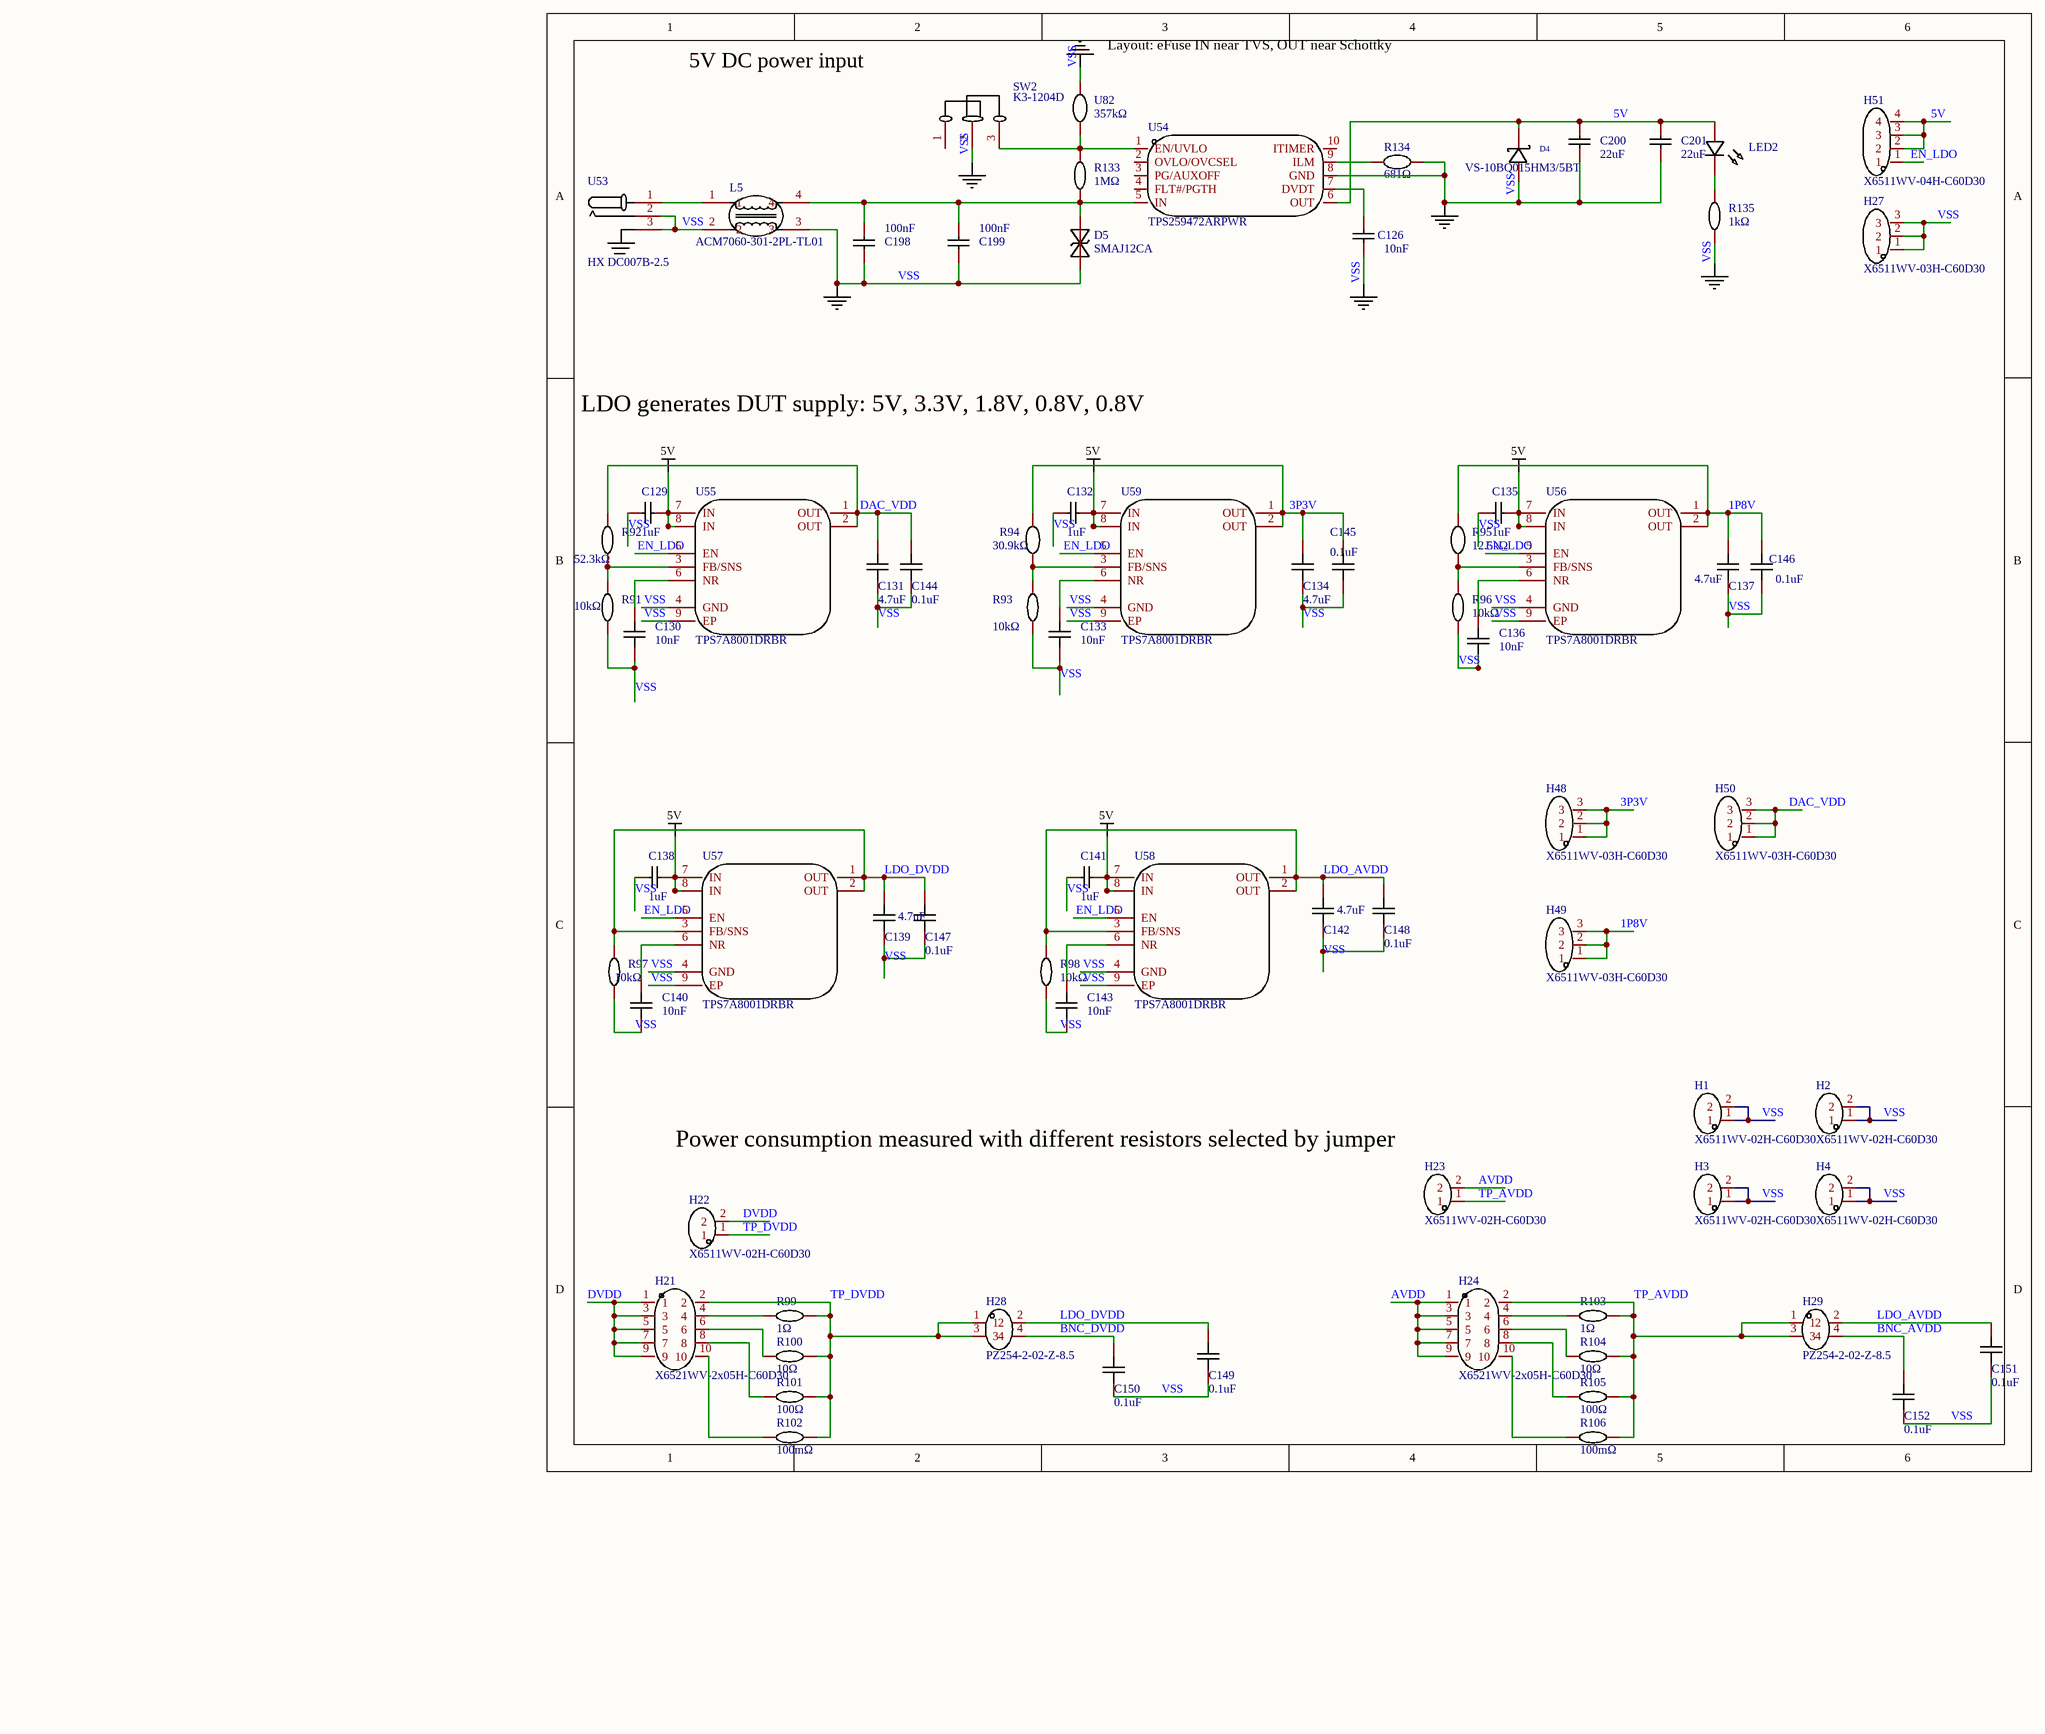
[diagram p0: MISC62793-2.schdoc]
# Altium project MISC62793-14.PrjPcb (part 1 of 4)
4 sheets, 201 parts. Net scope: global (net labels, ports and power ports of the same name join across sheets).
Board file: MISC62793.pcbdoc
Sheets:
  MISC62793-2.schdoc
  MISC62793-4.schdoc
  MISC62793-6.schdoc
  MISC62793-8.schdoc

## Sheet MISC62793-2.schdoc
size 279 x 274 mm; SheetNumber: 1; SheetTotal: 4

### Parts
C126  10nF  [C0603]
C129  1uF  [C0603]
C130  10nF  [C0603]
C131  4.7uF  [C0805]
C132  1uF  [C0603]
C133  10nF  [C0603]
C134  4.7uF  [C0805]
C135  1uF  [C0603]
C136  10nF  [C0603]
C137  4.7uF  [C0805]
C138  1uF  [C0603]
C139  4.7uF  [C0805]
C140  10nF  [C0603]
C141  1uF  [C0603]
C142  4.7uF  [C0805]
C143  10nF  [C0603]
C144  0.1uF  [C0402]
C145  0.1uF  [C0402]
C146  0.1uF  [C0402]
C147  0.1uF  [C0402]
C148  0.1uF  [C0402]
C149  0.1uF  [C0402]
C150  0.1uF  [C0402]
C151  0.1uF  [C0402]
C152  0.1uF  [C0402]
C198  100nF  [C0402]
C199  100nF  [C0402]
C200  22uF  [C1206]
C201  22uF  [C1206]
D4  VS-10BQ015HM3/5BT  [SMB_L4.6-W3.6-LS5.3-RD]
D5  SMAJ12CA  [SMA_L4.2-W2.7-LS5.0-BI]
H1  X6511WV-02H-C60D30  [HDR-TH_2P-P2.54-V-M]
H2  X6511WV-02H-C60D30  [HDR-TH_2P-P2.54-V-M]
H3  X6511WV-02H-C60D30  [HDR-TH_2P-P2.54-V-M]
H4  X6511WV-02H-C60D30  [HDR-TH_2P-P2.54-V-M]
H21  X6521WV-2x05H-C60D30  [HDR-TH_10P-P2.54-V-M-R2-C5-S2.54]
H22  X6511WV-02H-C60D30  [HDR-TH_2P-P2.54-V-M]
H23  X6511WV-02H-C60D30  [HDR-TH_2P-P2.54-V-M]
H24  X6521WV-2x05H-C60D30  [HDR-TH_10P-P2.54-V-M-R2-C5-S2.54]
H27  X6511WV-03H-C60D30  [HDR-TH_3P-P2.54-V-M]
H28  PZ254-2-02-Z-8.5  [HDR-TH_4P-P2.54-V-M-R2-C2-S2.54]
H29  PZ254-2-02-Z-8.5  [HDR-TH_4P-P2.54-V-M-R2-C2-S2.54]
H48  X6511WV-03H-C60D30  [HDR-TH_3P-P2.54-V-M]
H49  X6511WV-03H-C60D30  [HDR-TH_3P-P2.54-V-M]
H50  X6511WV-03H-C60D30  [HDR-TH_3P-P2.54-V-M]
H51  X6511WV-04H-C60D30  [HDR-TH_4P-P2.54-V-M]
L5  ACM7060-301-2PL-TL01  [FILTER-SMD_4P-L7.0-W6.0-TL_SMCM7060]
LED2  LED_0805-R  [LED_0805]  (value not drawn)
R91  10kΩ  [R0603]
R92  52.3kΩ  [R0603]
R93  10kΩ  [R0603]
R94  30.9kΩ  [R0603]
R95  12.5kΩ  [R0603]
R96  10kΩ  [R0603]
R97  10kΩ  [R0603]
R98  10kΩ  [R0603]
R99  1Ω  [R1206]
R100  10Ω  [R1206]
R101  100Ω  [R1206]
R102  100mΩ  [R1206]
R103  1Ω  [R1206]
R104  10Ω  [R1206]
R105  100Ω  [R1206]
R106  100mΩ  [R1206]
R133  1MΩ  [R1206]
R134  681Ω  [R0603]
R135  1kΩ  [R0805]
SW2  K3-1204D  [SW-TH_K3-1204D]
U53  HX DC007B-2.5  [DC-IN-TH_HX-DC007B-2.5]
U54  TPS259472ARPWR  [VQFN-10_L2.0-W2.0-P0.45-TL]
U55  TPS7A8001DRBR  [VSON-8_L3.0-W3.0-P0.65-TL-EP]
U56  TPS7A8001DRBR  [VSON-8_L3.0-W3.0-P0.65-TL-EP]
U57  TPS7A8001DRBR  [VSON-8_L3.0-W3.0-P0.65-TL-EP]
U58  TPS7A8001DRBR  [VSON-8_L3.0-W3.0-P0.65-TL-EP]
U59  TPS7A8001DRBR  [VSON-8_L3.0-W3.0-P0.65-TL-EP]
U82  357kΩ  [R1206]

### Nets
5V: C129.2 C132.2 C135.2 C138.2 C141.2 C200.2 C201.2 D4.1(C) H51.2 H51.3 H51.4 LED2.2(A) U54.6(OUT) U55.7(IN) U55.8(IN) U56.7(IN) U56.8(IN) U57.7(IN) U57.8(IN) U58.7(IN) U58.8(IN) U59.7(IN) U59.8(IN)
VSS: C126.1 C129.1 C130.1 C131.1 C132.1 C133.1 C134.1 C135.1 C136.1 C137.1 C138.1 C139.1 C140.1 C141.1 C142.1 C143.1 C144.1 C145.1 C146.1 C147.1 C148.1 C149.1 C150.1 C151.1 C152.1 C198.1 C199.1 C200.1 C201.1 D4.2(A) D5.1 H1.1 H1.2 H2.1 H2.2 H3.1 H3.2 H4.1 H4.2 H27.1 H27.2 H27.3 L5.2 L5.3 R91.1 R93.1 R96.1 R97.1 R98.1 R134.2 R135.1 SW2.2 U53.2 U53.3 U54.8(GND) U55.4(GND) U55.9(EP) U56.4(GND) U56.9(EP) U57.4(GND) U57.9(EP) U58.4(GND) U58.9(EP) U59.4(GND) U59.9(EP) U82.2
1P8V: C137.2 C146.2 H49.1 H49.2 H49.3 R95.2 U56.1(OUT) U56.2(OUT)
3P3V: C134.2 C145.2 H48.1 H48.2 H48.3 R94.1 U59.1(OUT) U59.2(OUT)
AVDD: H23.2 H24.1 H24.3 H24.5 H24.7 H24.9
BNC_AVDD: C152.2 H29.4
BNC_DVDD: C150.2 H28.4
DAC_VDD: C131.2 C144.2 H50.1 H50.2 H50.3 R92.2 U55.1(OUT) U55.2(OUT)
DVDD: H21.1 H21.3 H21.5 H21.7 H21.9 H22.2
EN_LDO: H51.1 U55.5(EN) U56.5(EN) U57.5(EN) U58.5(EN) U59.5(EN)
LDO_AVDD: C142.2 C148.2 C151.2 H29.2 R98.2 U58.1(OUT) U58.2(OUT) U58.3(FB/SNS)
LDO_DVDD: C139.2 C147.2 C149.2 H28.2 R97.2 U57.1(OUT) U57.2(OUT) U57.3(FB/SNS)
TP_AVDD: H23.1 H24.2 H29.1 H29.3 R103.2 R104.2 R105.2 R106.2
TP_DVDD: H21.2 H22.1 H28.1 H28.3 R99.2 R100.2 R101.2 R102.2
NetC126_2: C126.2 U54.7(DVDT)
NetC130_2: C130.2 U55.6(NR)
NetC133_2: C133.2 U59.6(NR)
NetC136_2: C136.2 U56.6(NR)
NetC140_2: C140.2 U57.6(NR)
NetC143_2: C143.2 U58.6(NR)
NetC198_2: C198.2 C199.2 D5.2 L5.4 R133.1 U54.5(IN)
NetH21_4: H21.4 R99.1
NetH21_6: H21.6 R100.1
NetH21_8: H21.8 R101.1
NetH21_10: H21.10 R102.1
NetH24_4: H24.4 R103.1
NetH24_6: H24.6 R104.1
NetH24_8: H24.8 R105.1
NetH24_10: H24.10 R106.1
NetL5_1: L5.1 U53.1
NetLED2_1: LED2.1(C) R135.2
NetR91_2: R91.2 R92.1 U55.3(FB/SNS)
NetR93_2: R93.2 R94.2 U59.3(FB/SNS)
NetR95_1: R95.1 R96.2 U56.3(FB/SNS)
NetR133_2: R133.2 SW2.3 U54.1(EN/UVLO) U82.1
NetR134_1: R134.1 U54.9(ILM)

Not connected (* = marked no-connect by the designer): SW2 1; U54 2(OVLO/OVCSEL) 3(PG/AUXOFF) 4(FLT#/PGTH) 10(ITIMER)

### Notes on the sheet
- 5V DC power input
- (near U82) Layout: eFuse IN near TVS, OUT near Schottky
- LDO generates DUT supply: 5V, 3.3V, 1.8V, 0.8V, 0.8V
- (near H23) Power consumption measured with different resistors selected by jumper

### Library data of the parts
C126 = CC0603KRX7R9BB103: Manufacturer: YAGEO(国巨); Add into BOM: yes; Tolerance: ±10%; Voltage Rated: 50V; Temperature Coefficient: X7R; Name: 10nF; Symbol: CC0603KRX7R9BB103; Device: CC0603KRX7R9BB103; Supplier: LCSC; Manufacturer Part: CC0603KRX7R9BB103; Value: 10nF; Supplier Part: C100042; JLCPCB Part Class: Extended Part; LCSC Part Name: 10nF ±10% 50V; Supplier Footprint: 0603; Datasheet: https://example.com/upload/public/pdf/source/20181008/C309510_22F155564471FAF6A489F7D68F34234E.pdf; Convert to PCB: yes
C129 C132 C135 C138 C141 = CL10A105KO8NNNC: Manufacturer: SAMSUNG(三星); Add into BOM: yes; Tolerance: ±10%; Voltage Rated: 16V; Temperature Coefficient: X5R; Name: 1uF; Symbol: CL10A105KO8NNNC; Device: CL10A105KO8NNNC; LCSC Part Name: 1uF ±10% 16V; Supplier Part: C1592; Manufacturer Part: CL10A105KO8NNNC; Supplier Footprint: 0603; JLCPCB Part Class: JLCPCB Part Class: Extended library; Datasheet: https://example.com/upload/public/pdf/source/20220919/9FBE606BE0D9532D730F292EB26DC5BB.pdf; Supplier: LCSC; Convert to PCB: yes; Value: 1uF
C130 C133 C136 C140 C143 = CC0603JRX7R7BB103: Manufacturer: YAGEO(国巨); Add into BOM: yes; Tolerance: ±5%; Voltage Rated: 16V; Temperature Coefficient: X7R; Name: 10nF; Symbol: CC0603JRX7R7BB103; Device: CC0603JRX7R7BB103; Supplier: LCSC; Supplier Part: C519509; Manufacturer Part: CC0603JRX7R7BB103; Value: 10nF; JLCPCB Part Class: JLCPCB Part Class: Extended library; LCSC Part Name: 10nF ±5% 16V; Supplier Footprint: 0603; Datasheet: https://example.com/upload/public/pdf/source/20200423/C519509_6D1EAA88CC7B3AD96A8CB6B0083D8E58.pdf; Convert to PCB: yes
C131 C134 C137 C139 C142 C144-C152 = C1210X475J5RAC7800: Manufacturer: KEMET(基美); Add into BOM: yes; Tolerance: ±5%; Voltage Rated: 50V; Temperature Coefficient: X7R; Symbol: C1210X475J5RAC7800; Device: C1210X475J5RAC7800; LCSC Part Name: 4.7uF ±5% 50V; Supplier Part: C600147; Manufacturer Part: C1210X475J5RAC7800; Supplier Footprint: 1210; JLCPCB Part Class: JLCPCB Part Class: Extended library; Datasheet: https://example.com/upload/public/pdf/source/20200618/C599807_353B987A11EFB304991393FBC85C4A7E.pdf; Supplier: LCSC; Convert to PCB: yes
  C131 C134 C137 C139 C142: Name: 4.7uF; Value: 4.7uF
  C144-C152: Name: 0.1uF; Value: 0.1uF
C198 C199 = CL05B104KO5NNNC: Manufacturer: SAMSUNG(三星); Add into BOM: yes; Tolerance: ±10%; Voltage Rated: 16V; Temperature Coefficient: X7R; Name: 100nF; Symbol: CL05B104KO5NNNC; Device: CL05B104KO5NNNC; Supplier: LCSC; Manufacturer Part: CL05B104KO5NNNC; Value: 100nF; Supplier Part: C1525; JLCPCB Part Class: JLCPCB Part Class: Basic library; LCSC Part Name: 100nF ±10% 16V; Supplier Footprint: 0402; Datasheet: https://example.com/upload/public/pdf/source/20160218/1457707763339.pdf; Convert to PCB: yes
C200 C201 = CL31A226KAHNNNE: Manufacturer: SAMSUNG(三星); Add into BOM: yes; Tolerance: ±10%; Voltage Rated: 25V; Temperature Coefficient: X5R; Name: 22uF; Symbol: CL31A226KAHNNNE; Device: CL31A226KAHNNNE; Supplier: LCSC; Manufacturer Part: CL31A226KAHNNNE; Value: 22uF; Supplier Part: C12891; JLCPCB Part Class: JLCPCB Part Class: Basic library; LCSC Part Name: 22uF ±10% 25V; Supplier Footprint: 1206; Datasheet: https://example.com/upload/public/pdf/source/20160218/1457707763339.pdf; Convert to PCB: yes
D4 = VS-10BQ015HM3/5BT: Manufacturer: VISHAY(威世); Add into BOM: yes; Forward Voltage (Vf@If): 210mV@1A; Reverse Voltage (Vr): 15V; Average Rectified Current (Io): 1A; Reverse Leakage Current (Ir): 500uA@15V; Name: VS-10BQ015HM3/5BT; Symbol: VS-10BQ015HM3/5BT; Device: VS-10BQ015HM3/5BT; Supplier: LCSC; Supplier Part: C413465; Manufacturer Part: VS-10BQ015HM3/5BT; JLCPCB Part Class: JLCPCB Part Class: Extended library; LCSC Part Name: 电压:15V 电流:1A; Supplier Footprint: DO-214AA(SMB); Datasheet: https://example.com/upload/public/pdf/source/20190819/C413465_3D2B1A8C7366D4425AB887DF85498F89.pdf; Convert to PCB: yes
D5 = SMAJ12CA_C908818: Manufacturer: GOODWORK(固得沃克); Add into BOM: yes; Reverse Stand-Off Voltage (Vrwm): 12V; Maximum Clamping Voltage: 19.9V; Peak Pulse Current (Ipp)@10/1000us: 20.1A; Breakdown Voltage: 13.3V; Reverse Leakage Current (Ir): 5uA; Type: TVS; Name: SMAJ12CA; Symbol: SMAJ12CA_C908818; Device: SMAJ12CA_C908818; Supplier: LCSC; Supplier Part: C908818; Manufacturer Part: SMAJ12CA; JLCPCB Part Class: JLCPCB Part Class: Extended library; LCSC Part Name: 双向TVS 12V截止 20.1A峰值脉冲; Supplier Footprint: SMA(DO-214AC); Datasheet: https://example.com/upload/public/pdf/source/20201231/C908757_5436EAF671B686EFC2F0DD2098F0ED89.pdf; Convert to PCB: yes
H1-H4 H22 H23 = X6511WV-02H-C60D30: Manufacturer: XKB Connection(中国星坤); Symbol: X6511WV-02H-C30D60; Add into BOM: yes; Pin Structure: 1x2P; Pitch: 2.54mm; Circluar Pins/Square Pins: Square pin; Current Rating (Max): 3A; Voltage Rating (Max): 250V; Soldering Temperature(Max): 260℃; Name: X6511WV-02H-C60D30; Device: X6511WV-02H-C60D30; LCSC Part Name: 1x2P 间距:2.54mm 方针; Supplier Part: C706874; Manufacturer Part: X6511WV-02H-C60D30; Supplier Footprint: 插件,P=2.54mm; JLCPCB Part Class: JLCPCB Part Class: Extended library; Supplier: LCSC; Convert to PCB: yes; Row Spacing: 2.54mm; Mounting Type: -; Number of Rows: Single row; Number of Pins: 2P; Length of Mating Pin: 6mm; Insulation Height: 2.5mm; Length of End Connection Pin: 3mm; Contact Material: Brass; Contact Plating: Gold; Operating Temperature Range: -40℃~+105℃; Color: Black
H21 H24 = X6521WV-2x05H-C60D30: Manufacturer: XKB Connection(中国星坤); Symbol: X6521WV-2×05H-C30D60; Add into BOM: yes; Pin Structure: 2x5P; Pitch: 2.54mm; Circluar Pins/Square Pins: Square pin; Current Rating (Max): 3A; Voltage Rating (Max): 250V; Soldering Temperature(Max): 260℃; Name: X6521WV-2x05H-C60D30; Device: X6521WV-2x05H-C60D30; LCSC Part Name: 2x5P 间距:2.54mm 方针; Supplier Part: C706895; Manufacturer Part: X6521WV-2x05H-C60D30; Supplier Footprint: 插件,P=2.54mm; JLCPCB Part Class: JLCPCB Part Class: Extended library; Datasheet: https://example.com/upload/public/pdf/source/20211009/DE33EBA4104B5B447A7BD8383FBBA145.pdf; Supplier: LCSC; Convert to PCB: yes; Row Spacing: 2.54mm; Mounting Type: -; Number of Rows: Dual row; Number of Pins: 10P; Length of Mating Pin: 6mm; Insulation Height: 2.5mm; Length of End Connection Pin: 3mm; Contact Material: Brass; Contact Plating: Gold; Operating Temperature Range: -40℃~+105℃; Color: Black
H27 H48-H50 = X6511WV-03H-C60D30: Manufacturer: XKB Connection(中国星坤); Symbol: X6511WV-03H-C30D60; Add into BOM: yes; Pin Structure: 1x3P; Pitch: 2.54mm; Circluar Pins/Square Pins: Square pin; Current Rating (Max): 3A; Voltage Rating (Max): 250V; Soldering Temperature(Max): 260℃; Name: X6511WV-03H-C60D30; Device: X6511WV-03H-C60D30; LCSC Part Name: 1x3P 间距:2.54mm 方针; Supplier Part: C706875; Manufacturer Part: X6511WV-03H-C60D30; Supplier Footprint: 插件,P=2.54mm; JLCPCB Part Class: JLCPCB Part Class: Extended library; Datasheet: https://example.com/upload/public/pdf/source/20221108/2FDDF9C694C8EDC81165E23F2EAAE597.pdf; Supplier: LCSC; Convert to PCB: yes; Row Spacing: -; Mounting Type: -; Number of Rows: Single row; Number of Pins: 3P; Length of Mating Pin: 6mm; Insulation Height: 2.5mm; Length of End Connection Pin: 3mm; Contact Material: Brass; Contact Plating: Gold; Operating Temperature Range: -40℃~+105℃; Color: Black
H28 H29 = PZ254-2-02-Z-8.5_C2894963: Manufacturer: HCTL(华灿天禄); Add into BOM: yes; Pin Structure: 2x2P; Pitch: 2.54mm; Circluar Pins/Square Pins: Square pin; Current Rating (Max): 3A; Soldering Temperature(Max): 260℃@10S; Name: PZ254-2-02-Z-8.5; Symbol: PZ254-2-02-Z-8.5; Device: PZ254-2-02-Z-8.5_C2894963; LCSC Part Name: 2x2P 间距:2.54mm 方针 直插; Supplier Part: C2894963; Manufacturer Part: PZ254-2-02-Z-8.5; Supplier Footprint: 插件,P=2.54mm; JLCPCB Part Class: JLCPCB Part Class: Extended library; Datasheet: https://example.com/upload/public/pdf/source/20230609/5BA09C8BEB9B31376F8BF6032FF67CAC.pdf; Supplier: LCSC; Convert to PCB: yes; Row Spacing: 2.54mm; Mounting Type: Through hole; Number of Rows: Dual row; Number of Pins: 4P; Voltage Rating (Max): -; Length of Mating Pin: 6mm; Insulation Height: 2.5mm; Length of End Connection Pin: 3mm; Contact Material: Brass; Operating Temperature Range: -40℃~+105℃; Color: Black
H51 = X6511WV-04H-C60D30: Manufacturer: XKB Connection(中国星坤); Symbol: X6511WV-04H-C30D60; Add into BOM: yes; Pin Structure: 1x4P; Pitch: 2.54mm; Circluar Pins/Square Pins: Square pin; Current Rating (Max): 3A; Voltage Rating (Max): 250V; Soldering Temperature(Max): 260℃; Name: X6511WV-04H-C60D30; Device: X6511WV-04H-C60D30; LCSC Part Name: 1x4P 间距:2.54mm 方针; Supplier Part: C706876; Manufacturer Part: X6511WV-04H-C60D30; Supplier Footprint: 插件,P=2.54mm; JLCPCB Part Class: JLCPCB Part Class: Extended library; Datasheet: https://example.com/upload/public/pdf/source/20211009/D19569EFFEB9776B42364DF7D41FD96A.pdf; Supplier: LCSC; Convert to PCB: yes; Row Spacing: 2.54mm; Mounting Type: -; Number of Rows: Single row; Number of Pins: 4P; Length of Mating Pin: 6mm; Insulation Height: 2.5mm; Length of End Connection Pin: 3mm; Contact Material: Brass; Contact Plating: Gold; Operating Temperature Range: -40℃~+105℃; Color: Black
L5 = ACM7060-301-2PL-TL01: Manufacturer: TDK; Value: 300Ω; Add into BOM: yes; Number of Lines: 2; Current Rating: 5A; Voltage Rating - DC: 80V; Impedance @ Frequency: 300Ω@100MHz; DC Resistance (DCR): 10mΩ; Name: ACM7060-301-2PL-TL01; Symbol: ACM7060-301-2PL-TL01; Device: ACM7060-301-2PL-TL01; Supplier: LCSC; Manufacturer Part: ACM7060-301-2PL-TL01; Supplier Part: C76580; JLCPCB Part Class: JLCPCB Part Class: Extended library; LCSC Part Name: 两路 贴片共模滤波器 阻抗300Ω@100MHz; Supplier Footprint: SMD,7x6mm; Datasheet: https://example.com/upload/public/pdf/source/20160918/1474166841345.pdf; Convert to PCB: yes; Operating Temperature: -40℃~+85℃
LED2 = LED_0805-R: Symbol: LED_R; Convert to PCB: yes; Device: LED_0805-R; Add into BOM: yes; Supplier Footprint: 0805
R91 R93 R96-R98 = 0603WAF1002T5E: Manufacturer: UNI-ROYAL(厚声); Add into BOM: yes; Tolerance: ±1%; Power(Watts): 100mW; Overload Voltage (Max): 75V; Temperature Coefficient: ±100ppm/℃; Name: 10kΩ; Symbol: 0603WAF1002T5E; Device: 0603WAF1002T5E; Supplier: LCSC; Manufacturer Part: 0603WAF1002T5E; Supplier Part: C25804; Value: 10kΩ; LCSC Part Name: 厚膜电阻 10kΩ ±1% 100mW; Supplier Footprint: 0603; Datasheet: https://example.com/upload/public/pdf/source/20200306/C422600_1E6D84923E4A46A82E41ADD87F860B5C.pdf; Convert to PCB: yes; Type: Thick film resistor; Operating Temperature Range: -55℃~+155℃
R92 = 0603WAF5232T5E: Manufacturer: UNI-ROYAL(厚声); Add into BOM: yes; Tolerance: ±1%; Power(Watts): 100mW; Overload Voltage (Max): 75V; Temperature Coefficient: ±100ppm/℃; Name: 52.3kΩ; Symbol: 0603WAF5232T5E; Device: 0603WAF5232T5E; Supplier: LCSC; Manufacturer Part: 0603WAF5232T5E; Supplier Part: C23198; Value: 52.3kΩ; JLCPCB Part Class: JLCPCB Part Class: Extended library; LCSC Part Name: 52.3kΩ ±1% 100mW 厚膜电阻; Supplier Footprint: 0603; Datasheet: https://example.com/upload/public/pdf/source/20200306/C422600_1E6D84923E4A46A82E41ADD87F860B5C.pdf; Convert to PCB: yes; Type: Thick film resistor; Operating Temperature Range: -55℃~+155℃
R94 = FRC0603F3092TS: Manufacturer: FOJAN(富捷); Add into BOM: yes; Tolerance: ±1%; Power(Watts): 100mW; Overload Voltage (Max): 75V; Temperature Coefficient: ±100ppm/℃; Name: 30.9kΩ; Symbol: FRC0603F3092TS; Device: FRC0603F3092TS; Supplier: LCSC; Supplier Part: C2930090; Manufacturer Part: FRC0603F3092TS; Value: 30.9kΩ; JLCPCB Part Class: JLCPCB Part Class: Extended library; LCSC Part Name: 30.9kΩ ±1% 100mW 厚膜电阻; Supplier Footprint: 0603; Datasheet: https://example.com/upload/public/pdf/source/20211221/925EC7D7225764EE0046F22065062C87.pdf; Convert to PCB: yes; Type: Thick film resistor; Operating Temperature Range: -55℃~+155℃
R95 = 0402WGF1252TCE: Manufacturer: UNI-ROYAL(厚声); Add into BOM: yes; Tolerance: ±1%; Power(Watts): 62.5mW; Overload Voltage (Max): 50V; Temperature Coefficient: ±100ppm/℃; Name: 12.5kΩ; Symbol: 0402WGF1252TCE; Device: 0402WGF1252TCE; Supplier: LCSC; Supplier Part: C407720; Manufacturer Part: 0402WGF1252TCE; Value: 12.5kΩ; JLCPCB Part Class: JLCPCB Part Class: Extended library; LCSC Part Name: 12.5kΩ ±1% 62.5mW 厚膜电阻; Supplier Footprint: 0402; Datasheet: https://example.com/upload/public/pdf/source/20200306/C422600_1E6D84923E4A46A82E41ADD87F860B5C.pdf; Convert to PCB: yes; Type: Thick film resistor; Operating Temperature Range: -55℃~+155℃
R99 R103 = 1206W4F100KT5E: Manufacturer: UNI-ROYAL(厚声); Add into BOM: yes; Tolerance: ±1%; Power(Watts): 250mW; Overload Voltage (Max): 200V; Temperature Coefficient: ±800ppm/℃; Name: 1Ω; Symbol: 1206W4F100KT5E; Device: 1206W4F100KT5E; Supplier: LCSC; Manufacturer Part: 1206W4F100KT5E; Supplier Part: C17928; Value: 1Ω; JLCPCB Part Class: JLCPCB Part Class: Basic library; LCSC Part Name: 1Ω ±1% 250mW 厚膜电阻; Supplier Footprint: 1206; Datasheet: https://example.com/upload/public/pdf/source/20200306/C422600_1E6D84923E4A46A82E41ADD87F860B5C.pdf; Convert to PCB: yes; Type: Thick film resistor; Operating Temperature Range: -55℃~+155℃
R100 R104 = 1206W4F100JT5E: Manufacturer: UNI-ROYAL(厚声); Add into BOM: yes; Tolerance: ±1%; Power(Watts): 250mW; Overload Voltage (Max): 200V; Temperature Coefficient: ±400ppm/℃; Name: 10Ω; Symbol: 1206W4F100JT5E; Device: 1206W4F100JT5E; Supplier: LCSC; Manufacturer Part: 1206W4F100JT5E; Supplier Part: C17903; Value: 10Ω; JLCPCB Part Class: JLCPCB Part Class: Basic library; LCSC Part Name: 10Ω ±1% 250mW 厚膜电阻; Supplier Footprint: 1206; Datasheet: https://example.com/upload/public/pdf/source/20200306/C422600_1E6D84923E4A46A82E41ADD87F860B5C.pdf; Convert to PCB: yes; Type: Thick film resistor; Operating Temperature Range: -55℃~+155℃
R101 R105 = 1206W4F1000T5E: Manufacturer: UNI-ROYAL(厚声); Add into BOM: yes; Tolerance: ±1%; Power(Watts): 250mW; Overload Voltage (Max): 200V; Temperature Coefficient: ±100ppm/℃; Name: 100Ω; Symbol: 1206W4F1000T5E; Device: 1206W4F1000T5E; Supplier: LCSC; Manufacturer Part: 1206W4F1000T5E; Supplier Part: C17901; Value: 100Ω; JLCPCB Part Class: JLCPCB Part Class: Basic library; LCSC Part Name: 100Ω ±1% 250mW 厚膜电阻; Supplier Footprint: 1206; Datasheet: https://example.com/upload/public/pdf/source/20200306/C422600_1E6D84923E4A46A82E41ADD87F860B5C.pdf; Convert to PCB: yes; Type: Thick film resistor; Operating Temperature Range: -55℃~+155℃
R102 R106 = 1206W4F100LT5E: Manufacturer: UNI-ROYAL(厚声); Add into BOM: yes; Tolerance: ±1%; Power(Watts): 250mW; Overload Voltage (Max): 200V; Temperature Coefficient: ±800ppm/℃; Name: 100mΩ; Symbol: 1206W4F100LT5E; Device: 1206W4F100LT5E; Supplier: LCSC; Manufacturer Part: 1206W4F100LT5E; Supplier Part: C25334; Value: 100mΩ; JLCPCB Part Class: JLCPCB Part Class: Basic library; LCSC Part Name: 100mΩ ±1% 250mW 厚膜电阻; Supplier Footprint: 1206; Datasheet: https://example.com/upload/public/pdf/source/20200306/C422600_1E6D84923E4A46A82E41ADD87F860B5C.pdf; Convert to PCB: yes; Type: Thick film resistor; Operating Temperature Range: -55℃~+155℃
R133 = 1206W4F1004T5E: Manufacturer: UNI-ROYAL(厚声); Add into BOM: yes; Tolerance: ±1%; Power(Watts): 250mW; Overload Voltage (Max): 200V; Temperature Coefficient: ±100ppm/℃; Name: 1MΩ; Symbol: 1206W4F1004T5E; Device: 1206W4F1004T5E; Supplier: LCSC; Manufacturer Part: 1206W4F1004T5E; Supplier Part: C17927; Value: 1MΩ; JLCPCB Part Class: JLCPCB Part Class: Basic library; LCSC Part Name: 1MΩ ±1% 250mW 厚膜电阻; Supplier Footprint: 1206; Datasheet: https://example.com/upload/public/pdf/source/20200306/C422600_1E6D84923E4A46A82E41ADD87F860B5C.pdf; Convert to PCB: yes; Type: Thick film resistor; Operating Temperature Range: -55℃~+155℃
R134 = RT0603BRD07681RL: Manufacturer: YAGEO(国巨); Add into BOM: yes; Tolerance: ±0.1%; Power(Watts): 100mW; Overload Voltage (Max): 75V; Temperature Coefficient: ±25ppm/℃; Name: 681Ω; Symbol: RT0603BRD07681RL; Device: RT0603BRD07681RL; LCSC Part Name: 薄膜电阻 681Ω ±0.1% 100mW; Supplier Part: C705792; Manufacturer Part: RT0603BRD07681RL; Supplier Footprint: 0603; JLCPCB Part Class: JLCPCB Part Class: Extended library; Datasheet: https://example.com/upload/public/pdf/source/20200720/C705792_EDF314EE001EB4AE666F730223633204.pdf; Supplier: LCSC; Convert to PCB: yes; Type: Thin film resistor; Value: 681Ω; Operating Temperature Range: -55℃~+155℃
R135 = RT0805BRD071KL: Manufacturer: YAGEO(国巨); Add into BOM: yes; Tolerance: ±0.1%; Power(Watts): 125mW; Overload Voltage (Max): 150V; Temperature Coefficient: ±25ppm/℃; Name: 1kΩ; Symbol: RT0805BRD071KL; Device: RT0805BRD071KL; LCSC Part Name: 薄膜电阻 1kΩ ±0.1% 125mW; Supplier Part: C110774; Manufacturer Part: RT0805BRD071KL; Supplier Footprint: 0805; JLCPCB Part Class: JLCPCB Part Class: Extended library; Datasheet: https://example.com/upload/public/pdf/source/20171026/C133380_15089840010201058857.pdf; Supplier: LCSC; Convert to PCB: yes; Type: Thin film resistor; Value: 1kΩ; Operating Temperature Range: -55℃~+155℃
SW2 = K3-1204D: Manufacturer: 韩国韩荣; Add into BOM: yes; Circuit: SPDT; Pin Style: PC pin; Switch Length: 10mm; Switch Width: 2.5mm; Switch Height: 6mm; Actuator Color: Red; Current Rating (AC): 5A; Voltage Rating (AC): 120V; Mechanical Life: 5万次; Name: K3-1204D; Symbol: K3-1204D; Device: K3-1204D; LCSC Part Name: 直插双档 滑动开关; Supplier Part: C145861; Manufacturer Part: K3-1204D; Supplier Footprint: 插件; JLCPCB Part Class: JLCPCB Part Class: Extended library; Datasheet: https://example.com/upload/public/pdf/source/20210810/A7BCE8A3AE6875067403B729968221B7.pdf; Supplier: LCSC; Convert to PCB: yes; Actuator Style: -; Mounting Style: Through hole; Voltage Rating (DC): -; Operating Temperature: -25℃~+80℃
U53 = HX DC007B-2.5: Manufacturer: hanxia(韩下); Add into BOM: yes; Connector Type: Connector Type: DC power jack; Inside Contact Diameter: 2.5mm; Outside Contact Diameter: 6.4mm; Current Rating (Max): 7A; Voltage Rating (Max): 20V; Name: HX DC007B-2.5; Symbol: HX DC007B-2.5; Device: HX DC007B-2.5; Supplier: LCSC; Supplier Part: C19189083; Manufacturer Part: HX DC007B-2.5; LCSC Part Name: DC电源插座 内径:2.5mm 外径:6.4mm; Supplier Footprint: 插件; Datasheet: https://example.com/upload/public/pdf/source/20231103/814B3421283469BAAEFFF9B7A53EC0CB.pdf; Convert to PCB: yes; Mounting Style: Right angle; Operating Temperature Range: -25℃~+70℃
U54 = TPS259472ARPWR: Manufacturer: TI(德州仪器); Add into BOM: yes; Voltage Rating: 2.7V~23V; Name: TPS259472ARPWR; Symbol: TPS259472ARPWR; Device: TPS259472ARPWR; LCSC Part Name: TPS259472ARPWR; Supplier Part: C3662789; Manufacturer Part: TPS259472ARPWR; Supplier Footprint: VQFN-10-HR(2x2); JLCPCB Part Class: JLCPCB Part Class: Extended library; Supplier: LCSC; Convert to PCB: yes; Operating temperature: -40℃~+125℃
U55-U59 = TPS7A8001DRBR: Manufacturer: TI(德州仪器); Add into BOM: yes; Output Type: Adjustable; Maximum Input Voltage: 6.5V; Output Voltage: 800mV~6V; MAX Output Current: 1A; Power Supply Rejection Ratio (PSRR): 63dB; Dropout Voltage: 500mV@(1A); Output Polarity: Positive; Number of Outputs: 1; Name: TPS7A8001DRBR; Symbol: TPS7A8001DRBR; Device: TPS7A8001DRBR; LCSC Part Name: ADJ 输入6.5V 输出0.8V~6V 1A; Supplier Part: C105265; Manufacturer Part: TPS7A8001DRBR; Supplier Footprint: VSON-8-EP(3x3); JLCPCB Part Class: Extended Part; Supplier: LCSC; Convert to PCB: yes
U82 = RT1206BRD07357KL: Manufacturer: YAGEO(国巨); Add into BOM: yes; Tolerance: ±0.1%; Power(Watts): 250mW; Temperature Coefficient: ±25ppm/℃; Name: 357kΩ; Symbol: RT1206BRD07357KL; Device: RT1206BRD07357KL; LCSC Part Name: 薄膜电阻 357kΩ ±0.1% 250mW; Supplier Part: C870672; Manufacturer Part: RT1206BRD07357KL; Supplier Footprint: 1206; JLCPCB Part Class: JLCPCB Part Class: Extended library; Datasheet: https://example.com/upload/public/pdf/source/20200610/C326738_5639A9F1B6EB6E4AE2197577D3456E7F.pdf; Supplier: LCSC; Convert to PCB: yes; Type: Thin film resistor; Value: 357kΩ; Operating Temperature Range: -55℃~+155℃